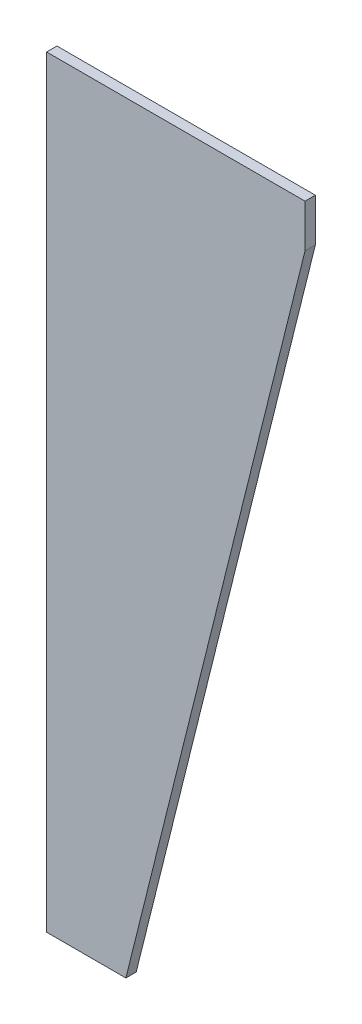
SolidWorks part; units mm, degrees
ref_plane "Front Plane" through (0, 0, 0) normal (0, 0, 1) x (1, 0, 0)
ref_plane "Top Plane" through (0, 0, 0) normal (0, 1, 0) x (1, 0, 0)
ref_plane "Right Plane" through (0, 0, 0) normal (1, 0, 0) x (0, 0, -1)
sketch "Sketch1" plane through (0, 0, 0) normal (0, 0, 1) x (1, 0, 0)
  line L0 (0, 0) -> (0, 885)
  line L1 (0, 885) -> (300, 885)
  line L2 (300, 885) -> (300, 835)
  line L3 (300, 835) -> (92, 0)
  line L4 (92, 0) -> (0, 0)
  dimension "D1" = 300
  dimension "D2" = 50
  dimension "D3" = 885
  dimension "D4" = 92
extrude "Boss-Extrude1" add sketch "Sketch1" along normal blind 12
